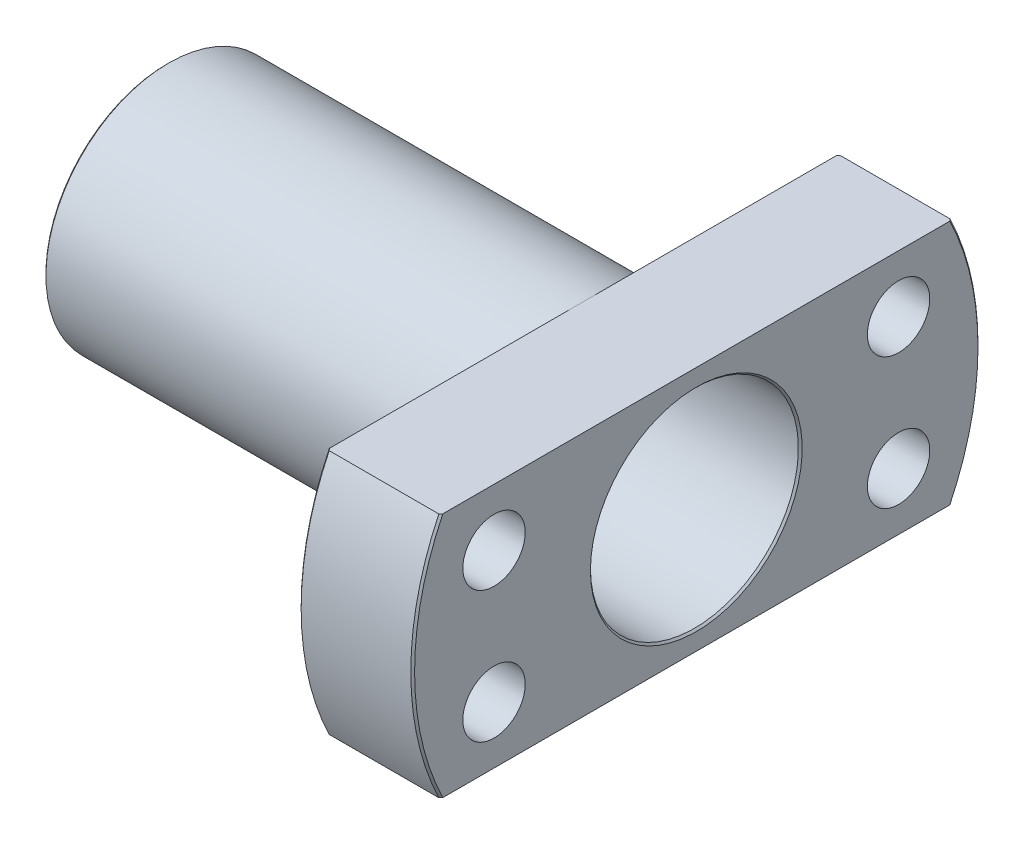
SolidWorks part; units mm, degrees
material "Q235-AF (Ni)"
ref_plane "Front Plane" through (0, 0, 0) normal (0, 0, 1) x (1, 0, 0)
ref_plane "Top Plane" through (0, 0, 0) normal (0, 1, 0) x (1, 0, 0)
ref_plane "Right Plane" through (0, 0, 0) normal (1, 0, 0) x (0, 0, -1)
sketch "Sketch1" plane through (0, 0, 0) normal (0, 0, 1) x (1, 0, 0)
  line L0 (0, 0) -> (104.7938, 0) construction
  line L1 (0, 0) -> (0, 13)
  line L2 (0, 13) -> (44, 13)
  line L3 (44, 13) -> (44, 30)
  line L4 (44, 30) -> (56, 30)
  line L5 (56, 30) -> (56, 11)
  line L6 (56, 11) -> (6, 11)
  line L7 (6, 11) -> (6, 0)
  line L8 (6, 0) -> (0, 0)
  dimension "D1" = 50
  dimension "D2" = 6
  dimension "D3" = 12
  dimension "D4" = 2
  dimension "D5" = 60
  dimension "D6" = 22
revolve "Revolve1" add sketch "Sketch1" angle 360 about L0
sketch "Sketch2" plane through (0, 0, 0) normal (-1, 0, 0) x (0, 0, 1)
  circle A0 centre (0, 0) radius 5.25
  dimension "D1" = 10.5
extrude "Cut-Extrude1" cut sketch "Sketch2" against normal through all
sketch "Sketch3" plane through (44, 0, 0) normal (-1, 0, 0) x (0, 0, 1)
  line L0 (27.037, 13) -> (-27.037, 13)
  line L1 (27.037, -13) -> (-27.037, -13)
  circle A0 centre (0, 0) radius 30 construction
  arc A1 (27.037, 13) -> (-27.037, 13) centre (0, 0) ccw
  arc A2 (-27.037, -13) -> (27.037, -13) centre (0, 0) ccw
  circle A3 centre (0, 0) radius 13 construction
extrude "Cut-Extrude2" cut sketch "Sketch3" against normal up to next
hole_wizard "Hole size per hex socket head cap screw type 1" positions "3DSketch1" profile "Sketch4" counterbore size "M6" standard "Gb" end condition through all
sketch3d "3DSketch1"
  line L0 (44, 0, 0) -> (0, 0, 0) construction
  line L1 (56, 0, 0) -> (44, 0, 0) construction
  line L2 (44, -6.9529, -21.3988) -> (44, 6.9529, -21.3988) construction
  line L4 (44, -6.9529, 21.3988) -> (44, 6.9529, 21.3988) construction
  line L6 (44, 0, -21.3988) -> (44, 0, 0) construction
  line L7 (44, 0, 0) -> (44, 0, 21.3988) construction
  line L8 (44, 0, 0) -> (44, -6.9529, -21.3988) construction
  line L10 (44, 0, 0) -> (44, 6.9529, -21.3988) construction
  line L12 (44, 0, 0) -> (44, 6.9529, 21.3988) construction
  line L14 (44, 0, 0) -> (44, -6.9529, 21.3988) construction
  circle A0 centre (44, 0, 0) radius 22.5
  point P0 (44, -6.9529, 21.3988)
  point P2 (44, 6.9529, 21.3988)
  point P4 (44, 6.9529, -21.3988)
  point P6 (44, -6.9529, -21.3988)
  point P10 (66.5, 0, 0)
  dimension "D1" = 45
  dimension "D2" = 36
sketch "Sketch4" plane through (44, -6.9529, 21.3988) normal (0, 1, 0) x (0, 0, 1)
  line L0 (0, 0) -> (0, 12)
  line L1 (0, 12) -> (3.3, 12)
  line L3 (3.3, 12) -> (3.3, 6.8)
  line L4 (3.3, 6.8) -> (5.5, 6.8)
  line L5 (5.5, 6.8) -> (5.5, 0)
  line L7 (5.5, 0) -> (0, 0)
  line L11 (0, -6.35) -> (0, 107.95) construction
  dimension "通孔孔直径" = 6.6
  dimension "通孔孔深度" = 12
  dimension "柱形沉头孔直径" = 11
  dimension "柱形沉头孔深度" = 6.8
chamfer "Chamfer1" distance 0.2 angle 45 6 edges at (44, 0, 30) (44, 0, -30) (56, 0, -30) (56, 0, 30) (0, 0, 5.25) (0, 0, 13)
chamfer "Chamfer2" distance 0.2 angle 45 1 edges at (56, 0, 11)
chamfer "Chamfer3" distance 1 angle 45 1 edges at (6, 0, 5.25)
